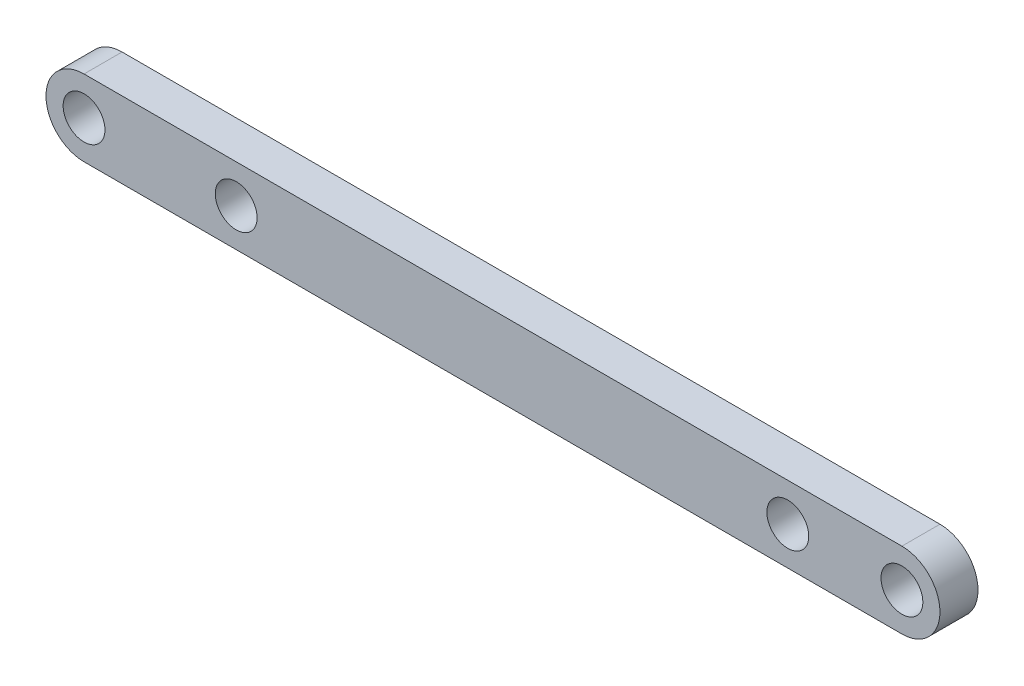
SolidWorks part; units mm, degrees
ref_plane "Alzado" through (0, 0, 0) normal (0, 0, 1) x (1, 0, 0)
ref_plane "Planta" through (0, 0, 0) normal (0, 1, 0) x (1, 0, 0)
ref_plane "Vista lateral" through (0, 0, 0) normal (1, 0, 0) x (0, 0, -1)
sketch "Sketch1" plane through (0, 0, 0) normal (0, 0, 1) x (1, 0, 0)
  line L0 (-10.75, 0) -> (10.75, 0) construction
  line L1 (-10.75, 1) -> (10.75, 1)
  line L2 (-10.75, -1) -> (10.75, -1)
  arc A0 (-10.75, 1) -> (-10.75, -1) centre (-10.75, 0) ccw
  arc A1 (10.75, -1) -> (10.75, 1) centre (10.75, 0) ccw
  circle A2 centre (-10.75, 0) radius 0.55
  circle A3 centre (10.75, 0) radius 0.55
  circle A4 centre (-6.75, 0) radius 0.55
  circle A5 centre (7.75, 0) radius 0.55
  point P3 (0, 0)
  dimension "D3" = 1.1
  dimension "D4" = 4
  dimension "D5" = 18.5
  dimension "D1" = 21.5
  dimension "D2" = 2
extrude "Thigh1 length" add sketch "Sketch1" along normal mid plane 1
sketch "Sketch2" plane through (0, 0, 0.5) normal (0, 0, 1) x (1, 0, 0)
  circle A0 centre (-10.75, 0) radius 1.55
  circle A1 centre (10.75, 0) radius 1.55
  circle A2 centre (-6.75, 0) radius 1.55
  dimension "D1" = 3.1
extrude "Cortar-Extruir1" [suppressed] cut sketch "Sketch2" against normal blind 1
